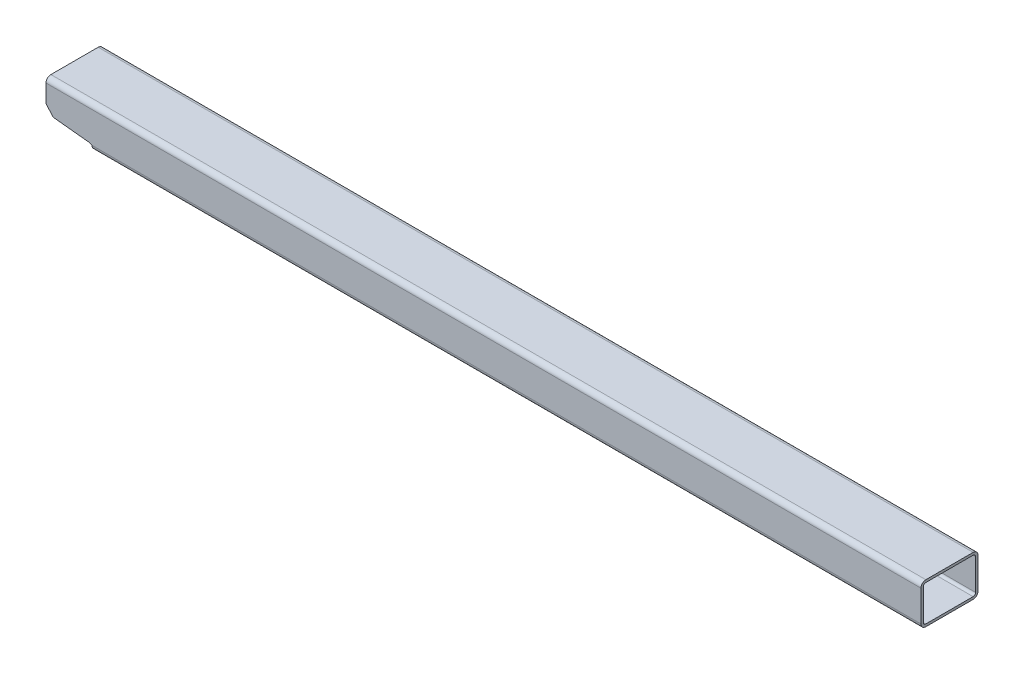
SolidWorks part; units mm, degrees
material "Q235B"
ref_plane "前视基准面" through (0, 0, 0) normal (0, 0, 1) x (1, 0, 0)
ref_plane "上视基准面" through (0, 0, 0) normal (0, 1, 0) x (1, 0, 0)
ref_plane "右视基准面" through (0, 0, 0) normal (1, 0, 0) x (0, 0, -1)
other "Configuration Table"
sketch "草图1" plane through (0, 0, 0) normal (0, 0, 1) x (1, 0, 0)
  line L0 (-569.75, 0) -> (569.75, 0)
  point P2 (0, 0)
  dimension "D1" = 1139.5
other "Gb／6728-1986矩形空心型钢 070 X 50 X 3(1)"
ref_plane "基准面1" through (-569.75, 0, 0) normal (1, 0, 0) x (0, 1, 0)
sketch "Sketch1" plane through (-569.75, 0, 0) normal (1, 0, 0) x (0, 1, 0)
  line L0 (-19, -32) -> (19, -32)
  line L1 (-22, -29) -> (-22, 29)
  line L2 (19, 32) -> (-19, 32)
  line L3 (22, 29) -> (22, -29)
  line L4 (-19, -35) -> (19, -35)
  line L5 (-25, -29) -> (-25, 29)
  line L6 (19, 35) -> (-19, 35)
  line L7 (25, 29) -> (25, -29)
  arc A0 (25, 29) -> (19, 35) centre (19, 29) ccw
  arc A1 (19, -35) -> (25, -29) centre (19, -29) ccw
  arc A2 (-25, -29) -> (-19, -35) centre (-19, -29) ccw
  arc A3 (-19, 35) -> (-25, 29) centre (-19, 29) ccw
  arc A4 (-19, 32) -> (-22, 29) centre (-19, 29) ccw
  arc A5 (22, 29) -> (19, 32) centre (19, 29) ccw
  arc A6 (19, -32) -> (22, -29) centre (19, -29) ccw
  arc A7 (-22, -29) -> (-19, -32) centre (-19, -29) ccw
  point P0 (0, 35)
  point P1 (25, 0)
  point P2 (0, -35)
  point P3 (-25, 0)
  point P4 (-25, 35)
  point P5 (25, 35)
  point P6 (25, -35)
  point P7 (-25, -35)
  point P8 (0, 0)
  point P33 (0, 0)
  dimension "D1" = 6
  dimension "Thickness" = 3
  dimension "V_leg" = 70
  dimension "H_leg" = 50
sketch "草图2" plane through (0, 0, -35) normal (0, 0, -1) x (-1, 0, 0)
  line L0 (513.25, -25) -> (513.25, -19)
  line L1 (-569.75, -19) -> (569.75, -19) construction
  line L2 (513.25, -19) -> (517.7274, -17.4986)
  line L3 (517.7274, -17.4986) -> (560.7953, -12.972)
  line L4 (560.7953, -12.972) -> (569.75, -3.0268)
  line L5 (569.75, -3.0268) -> (-2717.25, -3.0268) construction
  line L6 (569.75, -19) -> (569.75, 19) construction
  line L7 (569.75, -3.0268) -> (574.75, -3.0268)
  line L8 (574.75, -3.0268) -> (574.75, -30)
  line L9 (574.75, -30) -> (513.25, -30)
  line L10 (513.25, -30) -> (513.25, -25)
  line L11 (-569.75, -25) -> (569.75, -25) construction
  dimension "D1" = 5
  dimension "D2" = 5
extrude "切除-拉伸1" cut sketch "草图2" against normal through all and the other way through all
sketch "草图5" plane through (0, 0, 35) normal (0, 0, 1) x (1, 0, 0)
  line L0 (569.75, 19) -> (569.75, -19) construction
  line L1 (574.75, 30) -> (503.75, 30)
  line L2 (574.75, 30) -> (574.75, -30)
  line L3 (574.75, -30) -> (503.75, -30)
  line L4 (503.75, 30) -> (503.75, -30)
  line L5 (569.75, 25) -> (-569.75, 25) construction
  line L6 (569.75, -25) -> (-513.25, -25) construction
  dimension "D1" = 66
  dimension "D2" = 5
  dimension "D3" = 5
  dimension "D4" = 5
extrude "切除-拉伸4" cut sketch "草图5" against normal through all
